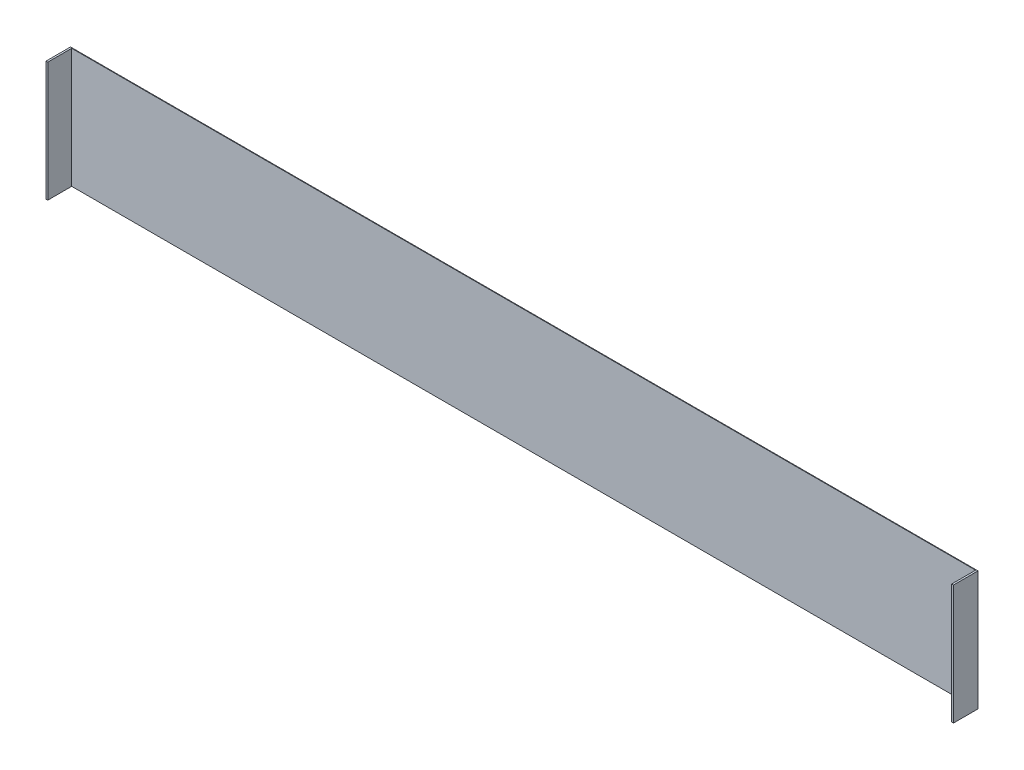
SolidWorks part; units mm, degrees
material "1060 合金"
ref_plane "前视基准面" through (0, 0, 0) normal (0, 0, 1) x (1, 0, 0)
ref_plane "上视基准面" through (0, 0, 0) normal (0, 1, 0) x (1, 0, 0)
ref_plane "右视基准面" through (0, 0, 0) normal (1, 0, 0) x (0, 0, -1)
other "Configuration Table"
sketch "草图1" plane through (0, 0, 0) normal (0, 0, 1) x (1, 0, 0)
  line L1 (-759, -100) -> (759, -100)
  line L2 (-759, -100) -> (-759, 100)
  line L3 (-759, 100) -> (759, 100)
  line L4 (759, -100) -> (759, 100)
  line L5 (-759, -100) -> (759, 100) construction
  line L6 (-759, 100) -> (759, -100) construction
  point P0 (0, 0)
  dimension "D1" = 1518
  dimension "D2" = 200
extrude "凸台-拉伸1" add sketch "草图1" along normal blind 1
sketch "草图2" plane through (0, 0, 1) normal (0, 0, 1) x (1, 0, 0)
  line L0 (-759, -100) -> (759, -100) construction
  line L1 (-759, 100) -> (-756, 100)
  line L2 (-759, 100) -> (-759, -100)
  line L3 (-759, -100) -> (-756, -100)
  line L4 (-756, 100) -> (-756, -100)
  dimension "D1" = 3
extrude "凸台-拉伸2" add sketch "草图2" along normal blind 40
mirror "镜向1" about plane through (0, 0, 0) normal (1, 0, 0) of "凸台-拉伸2"
